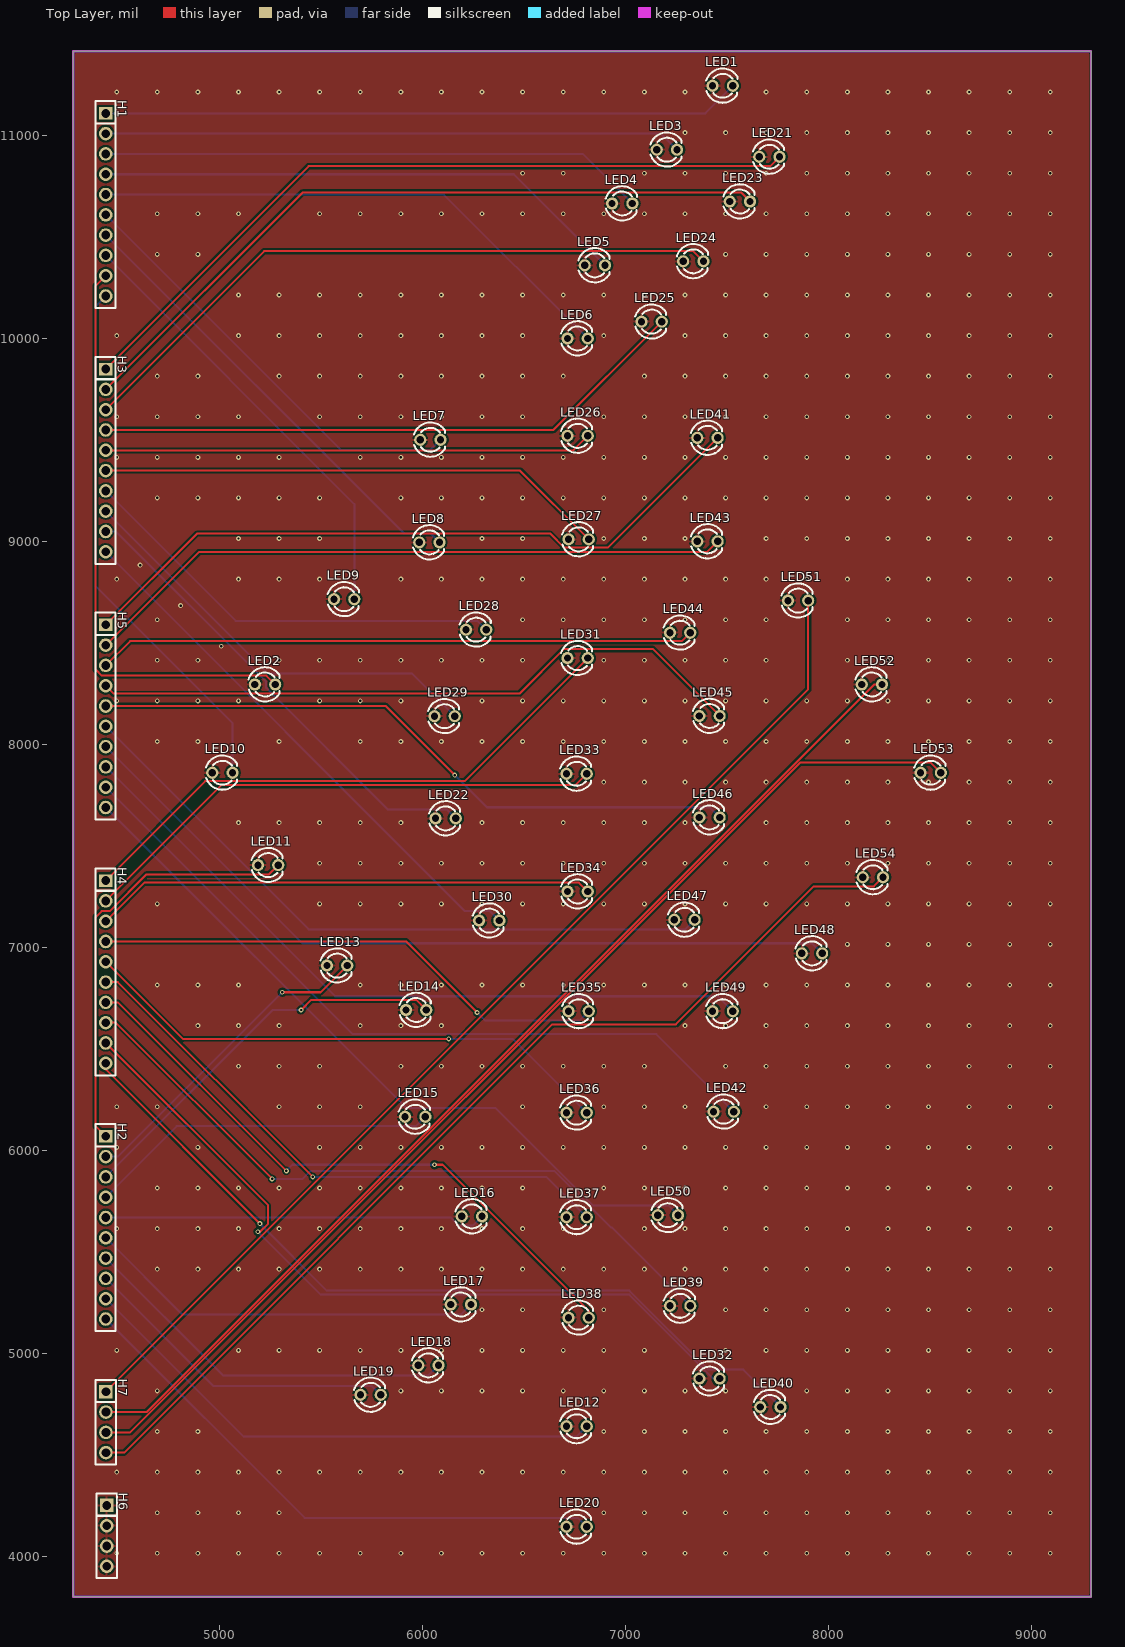
[diagram p0: Top Layer view]
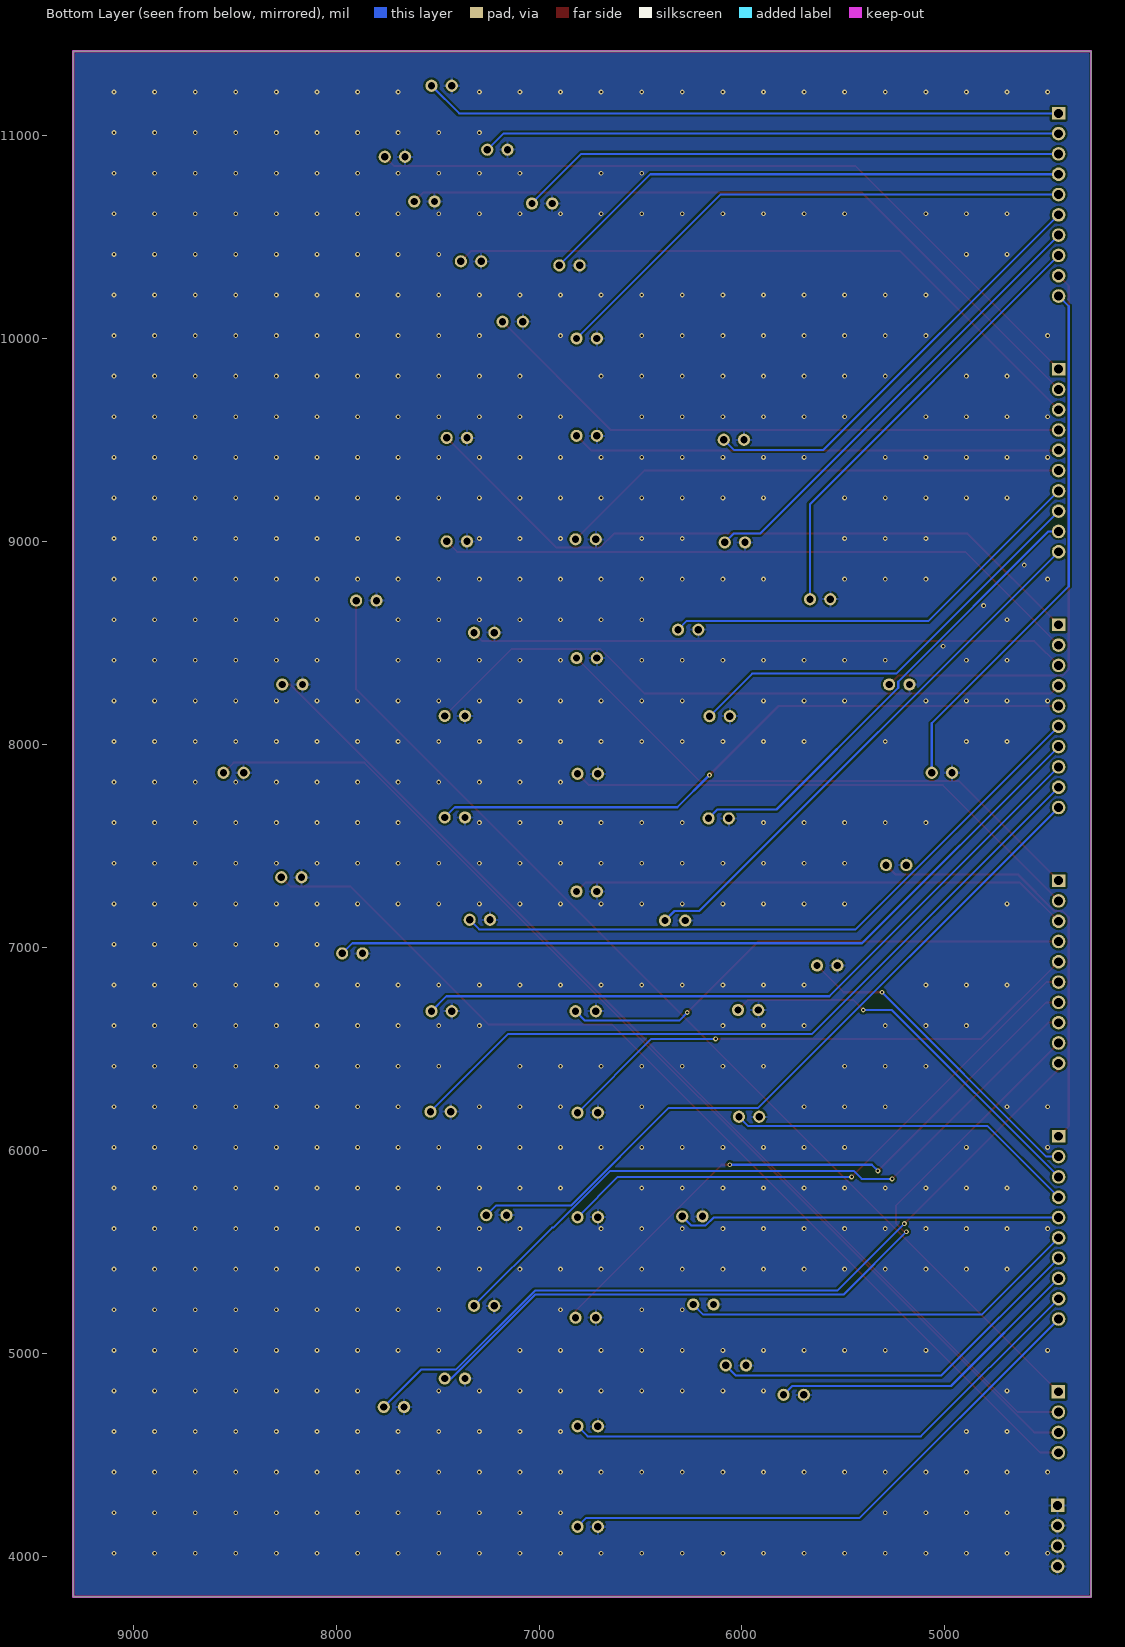
[diagram p1: Bottom Layer view, seen from below]
# Altium PCB MISC89091.pcbdoc
Units mil, origin at the board's own origin, x right, y up, seen from the top; angles counter-clockwise.
Board outline 5015 x 7615 mil, 2 copper layers (Top Layer, Bottom Layer), stack 62.206 mil thick; 61 components, 55 nets, 166 pads, 702 vias.

## Layer stack, top to bottom
Top Solder Mask Layer: solder mask 0.394, Dk 3.3
Top Layer: signal copper 1.379
Dielectric1: surface 59.449, FR4, Dk 4.5
Bottom Layer: signal copper 1.378
Bottom Solder Mask Layer: solder mask 0.394, Dk 3.3

## Board outline
4280,11415 4280,3800 9295,3800 9295,11415

## Design rules (kind name [scope] priority, off if disabled: settings)
BoardOutlineClearance copperThickness2oz_1 [All] p2 off: genericclearance=7.99 ignorepadtopadclearanceinfootprint=FALSE except(0: Arc-SplitContinuation Track-SplitContinuation SMDPad-SplitContinuation THPad-SplitContinuation Via-SplitContinuation Fill-SplitContinuation Region-SplitContinuation Poly-SplitContinuation Text-SplitContinuation Hole-SplitContinuation; 5.98: Arc-CutoutEdge SMDPad-CutoutEdge THPad-CutoutEdge Via-CutoutEdge Fill-CutoutEdge Region-CutoutEdge Text-CutoutEdge; 6.93: Hole-OutlineEdge Hole-CutoutEdge; 10: Poly-OutlineEdge Poly-CutoutEdge; 11.81: Arc-OutlineEdge Track-OutlineEdge SMDPad-OutlineEdge THPad-OutlineEdge Via-OutlineEdge Fill-OutlineEdge Region-OutlineEdge Text-OutlineEdge Track-CutoutEdge)
BoardOutlineClearance copperThickness1oz_1 [All] p4: genericclearance=4.02 ignorepadtopadclearanceinfootprint=FALSE except(0: Arc-SplitContinuation Track-SplitContinuation SMDPad-SplitContinuation THPad-SplitContinuation Via-SplitContinuation Fill-SplitContinuation Region-SplitContinuation Poly-SplitContinuation Text-SplitContinuation Hole-SplitContinuation; 6: SMDPad-CutoutEdge THPad-CutoutEdge Via-CutoutEdge Fill-CutoutEdge Region-CutoutEdge Text-CutoutEdge; 6.93: Hole-OutlineEdge Hole-CutoutEdge; 10: Poly-OutlineEdge Poly-CutoutEdge; 11.8: Arc-OutlineEdge Track-OutlineEdge SMDPad-OutlineEdge THPad-OutlineEdge Via-OutlineEdge Fill-OutlineEdge Region-OutlineEdge Text-OutlineEdge; 11.81: Arc-CutoutEdge Track-CutoutEdge)
Clearance copperThickness2oz [All] p1 off: gap=7.99 ignorepadtopadclearanceinfootprint=FALSE except(5.98: SMDPad-Track SMDPad-SMDPad THPad-Track SMDPad-THPad THPad-THPad Track-Via SMDPad-Via THPad-Via Via-Via Fill-Track Region-Track Fill-SMDPad Region-SMDPad Fill-THPad Region-THPad Fill-Via Region-Via Fill-Fill Fill-Region Region-Region Arc-Track Arc-SMDPad Arc-THPad Arc-Via Fill-Arc Region-Arc Arc-Arc Text-Track SMDPad-Text Text-THPad Text-Via Fill-Text Region-Text Arc-Text Text-Text; 6.93: Hole-Track Hole-SMDPad Hole-THPad Hole-Via Fill-Hole Region-Hole Hole-Arc Hole-Text; 10: Poly-Track Poly-SMDPad Poly-THPad Poly-Via Poly-Fill Poly-Region Poly-Poly Poly-Arc Poly-Text Poly-Hole)
Clearance copperThickness1oz [All] p3: gap=4.02 ignorepadtopadclearanceinfootprint=FALSE except(5.98: SMDPad-Track SMDPad-SMDPad THPad-Track SMDPad-THPad THPad-THPad Track-Via SMDPad-Via THPad-Via Via-Via Fill-Track Region-Track Fill-SMDPad Region-SMDPad Fill-THPad Region-THPad Fill-Via Region-Via Fill-Fill Fill-Region Region-Region; 6: Arc-Track Arc-SMDPad Arc-THPad Arc-Via Fill-Arc Region-Arc Arc-Arc Text-Track SMDPad-Text Text-THPad Text-Via Fill-Text Region-Text Arc-Text Text-Text; 6.93: Hole-Track Hole-SMDPad Hole-THPad Hole-Via Fill-Hole Region-Hole Hole-Arc Hole-Text; 10: Poly-Track Poly-SMDPad Poly-THPad Poly-Via Poly-Fill Poly-Region Poly-Poly Poly-Arc Poly-Text Poly-Hole)
Creepage creepage [All] p1: checkdistance=0 ignoreinternallayers=TRUE applytopolygonpour=TRUE
DiffPairsRouting differentialPair [All] p1: maxlimit=6 minlimit=6 mostfreqgap=6 toplayer_minwidth=5 toplayer_prefwidth=10 toplayer_maxwidth=100 toplayer_mingap=6 toplayer_prefgap=6 toplayer_maxgap=6 bottomlayer_minwidth=5 bottomlayer_prefwidth=10 bottomlayer_maxwidth=100 bottomlayer_mingap=6 bottomlayer_prefgap=6 bottomlayer_maxgap=6 maxuncoupledlength=10
HoleToHoleClearance otherClearance [All] p1: gap=11.81 allowstackedmicrovias=TRUE
Length netLength [All] p1: minlimit=0 maxlimit=0
MatchedLengths netLengthTolerance [All] p1: tolerance=1000
PasteMaskExpansion pasteMaskExpansion [All] p1: expansion=0
PlaneConnect innerPlane [All] p1: planeconnectstyle=Relief reliefexpansion=20 reliefentries=4 reliefconductorwidth=10 reliefairgap=10
PolygonConnect copperRegion [(InNet('P18') OR InNet('P19'))] p1: connectstyle=Relief reliefconductorwidth=10 reliefentries=4 polygonreliefangle="90 Angle" airgapwidth=10 via.connectstyle=Relief via.reliefconductorwidth=10 via.reliefentries=4 via.polygonreliefangle="90 Angle" via.airgapwidth=10
RoutingVias viaSize [All] p1: holewidth=12.01 width=24.02 viastyle="Through Hole" minholewidth=11.81 minwidth=19.68 maxholewidth=248.03 maxwidth=393.7
SolderMaskExpansion solderMaskExpansion [IsVia] p1: expansion=-1000 istentingtop=TRUE
SolderMaskExpansion solderMaskExpansion [All] p2: expansion=2 istentingtop=FALSE
Width copperThickness2oz_2 [All] p1 off: maxlimit=100 minlimit=8 preferedwidth=10
Width copperThickness1oz_2 [All] p2: maxlimit=100 minlimit=5 preferedwidth=10

## Components (designator, comment, footprint, x,y, rotation, side; value= is the part's Value field where it differs from the comment)
H1 "" HDR-TH_10P-P2.54-V-F 4440,10658.93 r270 top
H2 "" HDR-TH_10P-P2.54-V-F 4440,5618.53 r270 top
H3 "" HDR-TH_10P-P2.54-V-F 4440,9398.83 r270 top
H4 "" HDR-TH_10P-P2.54-V-F 4440,6878.63 r270 top
H5 "" HDR-TH_10P-P2.54-V-F 4440,8138.73 r270 top
H6 "" HDR-TH_4P-P2.54-V-F 4445,4100 r270 top
H7 "" HDR-TH_4P-P2.54-V-F 4440.79,4660 r270 top
LED1 "" LED_TH-3mm 7480,11245 r0 top
LED2 "" LED_TH-3mm 5225,8295 r0 top
LED3 "" LED_TH-3mm 7205,10930 r0 top
LED4 "" LED_TH-3mm 6985,10665 r0 top
LED5 "" LED_TH-3mm 6850,10360 r0 top
LED6 "" LED_TH-3mm 6765,10000 r0 top
LED7 "" LED_TH-3mm 6039.84,9500.65 r0 top
LED8 "" LED_TH-3mm 6035,8995 r0 top
LED9 "" LED_TH-3mm 5615,8715 r0 top
LED10 "" LED_TH-3mm 5015,7860 r0 top
LED11 "" LED_TH-3mm 5240,7405 r0 top
LED12 "" LED_TH-3mm 6760,4640 r0 top
LED13 "" LED_TH-3mm 5580,6910 r0 top
LED14 "" LED_TH-3mm 5969.37,6691.15 r0 top
LED15 "" LED_TH-3mm 5965,6165 r0 top
LED16 "" LED_TH-3mm 6244.37,5674.15 r0 top
LED17 "" LED_TH-3mm 6190,5240 r0 top
LED18 "" LED_TH-3mm 6030,4940 r0 top
LED19 "" LED_TH-3mm 5745,4795 r0 top
LED20 "" LED_TH-3mm 6760,4145 r0 top
LED21 "" LED_TH-3mm 7710,10895 r0 top
LED22 "" LED_TH-3mm 6114.68,7635.14 r0 top
LED23 "" LED_TH-3mm 7564.68,10674.65 r0 top
LED24 "" LED_TH-3mm 7335,10380 r0 top
LED25 "" LED_TH-3mm 7129.68,10082.65 r0 top
LED26 "" LED_TH-3mm 6765,9520 r0 top
LED27 "" LED_TH-3mm 6770,9010 r0 top
LED28 "" LED_TH-3mm 6265,8565 r0 top
LED29 "" LED_TH-3mm 6109.68,8138.65 r0 top
LED30 "" LED_TH-3mm 6329.68,7131.64 r0 top
LED31 "" LED_TH-3mm 6765,8425 r0 top
LED32 "" LED_TH-3mm 7415,4875 r0 top
LED33 "" LED_TH-3mm 6760,7855 r0 top
LED34 "" LED_TH-3mm 6765,7275 r0 top
LED35 "" LED_TH-3mm 6770,6685 r0 top
LED36 "" LED_TH-3mm 6760,6185 r0 top
LED37 "" LED_TH-3mm 6760,5670 r0 top
LED38 "" LED_TH-3mm 6770,5175 r0 top
LED39 "" LED_TH-3mm 7270.63,5233.65 r0 top
LED40 "" LED_TH-3mm 7715,4735 r0 top
LED41 "" LED_TH-3mm 7405,9510 r0 top
LED42 "" LED_TH-3mm 7485,6190 r0 top
LED43 "" LED_TH-3mm 7405,9000 r0 top
LED44 "" LED_TH-3mm 7270,8550 r0 top
LED45 "" LED_TH-3mm 7415,8140 r0 top
LED46 "" LED_TH-3mm 7415,7640 r0 top
LED47 "" LED_TH-3mm 7291.58,7135.65 r0 top
LED48 "" LED_TH-3mm 7920,6970 r0 top
LED49 "" LED_TH-3mm 7480,6685 r0 top
LED50 "" LED_TH-3mm 7210,5680 r0 top
LED51 "" LED_TH-3mm 7851.26,8708.22 r0 top
LED52 "" LED_TH-3mm 8215,8295 r0 top
LED53 "" LED_TH-3mm 8505,7860 r0 top
LED54 "" LED_TH-3mm 8220,7345 r0 top

## Footprints (in the part's own frame and the unit in brackets; to place one, negate y for a bottom-side part, rotate by r counter-clockwise, add the part's x,y. Pads: shape width x height; smd on the part's side, far side on the other; paste and mask are expansions set on the pad)
HDR-TH_4P-P2.54-V-F [mm]
  rect 1.7x1.7 hole 1.1: 1(-3.81,0)
  round 1.7 hole 1.1: 2(-1.27,0) 3(1.27,0) 4(3.81,0)
  silkscreen extent -5.29,-1.27 5.29,1.27
HDR-TH_10P-P2.54-V-F [mm]
  rect 1.575x1.7 hole 1.1: 1(-11.43,0)
  round 1.7 hole 1.1: 2(-8.89,0) 3(-6.35,0) 4(-3.81,0) 5(-1.27,0) 6(1.27,0) 7(3.81,0) 8(6.35,0) 9(8.89,0) 10(11.43,0)
  silkscreen extent -12.95,-1.25 12.95,1.25
LED_TH-3mm [mil]
  round 60 hole 36 paste+0 mask+2: 1(-50,0) 2(50,0)
  silkscreen extent -81,-84 72,85

## Via types
v1: diameter 24.02, hole 12, Top Layer to Bottom Layer, 702 vias

## Nets (pads, with @x,y where several pads share a name; then routed paths per layer and width w, separated by ;. In a path a pad name is that pad's centre, name@x,y a point inside that pad or via, vN(x,y) a via of type N, cw(c..) or ccw(c..) an arc to the next point about the centre after c; other vN are vias at no path point)
P10: H1.1 LED1.2 | length 3146.4
  Bottom Layer w10: H1.1 7393.93,11108.93 LED1.2
P11: H1.2 LED3.2 | length 2847.7
  Bottom Layer w10: H1.2 7176.07,11008.93 LED3.2
P12: H1.3 LED4.2 | length 2696
  Bottom Layer w10: H1.3 6791.07,10908.93 LED4.2
P13: H1.4 LED5.2 | length 2646
  Bottom Layer w10: H1.4 6451.07,10808.93 LED5.2
P14: H1.5 LED6.2 | length 2668.6
  Bottom Layer w10: H1.5 6106.07,10708.93 LED6.2
P15: H1.6 LED7.2 | length 2150.3
  Bottom Layer w10: H1.6 5598.28,9450.65 6039.84,9450.65 LED7.2
P16: H1.7 LED8.2 | length 2272.1
  Bottom Layer w10: H1.7 5910,9038.93 6041.07,9038.93 LED8.2
P17: H1.8 LED9.2 | length 2201.3
  Bottom Layer w10: H1.8 5665,9183.93 LED9.2
P18: H1.9 LED2.2 | length 2876.3
  Top Layer w10: H1.9 4390,10258.93 4390,8368.94 4420,8338.94 5231.06,8338.94 LED2.2
P19: H1.10 LED10.2 | length 2649.2
  Bottom Layer w10: H1.10 4390,10158.93 4390,8778.93 5065,8103.93 LED10.2
P20: H2.1 LED11.2 | length 2106.9
  Top Layer w10: H2.1 4390,6118.53 4390,7148.52 4420,7178.52 4460,7178.52 4640,7358.52 5243.53,7358.52 LED11.2
P21: H2.2 LED13.2 | length 1580
  Top Layer w10: v1(5310,6778.53) 5498.52,6778.53 LED13.2
  Bottom Layer w10: H2.2 4500,5968.53 v1(5310,6778.53)
P22: H2.3 LED14.2 | length 1961.5
  Top Layer w10: v1(5402.62,6691.15) 5452.62,6741.15 5969.37,6741.15 LED14.2
  Bottom Layer w10: H2.3 5262.62,6691.15 v1(5402.62,6691.15)
P23: H2.4 LED15.2 | length 1739.2
  Bottom Layer w10: H2.4 4790,6118.53 5968.53,6118.53 LED15.2
P24: H2.5 LED16.2 | length 1889.8
  Bottom Layer w10: H2.5 6140,5668.53 6180,5628.53 6248.75,5628.53 LED16.2
P25: H2.6 LED17.2 | length 1977.5
  Bottom Layer w10: H2.6 4818.53,5190 6190,5190 LED17.2
P26: H2.7 LED18.2 | length 1900.3
  Bottom Layer w10: H2.7 5018.53,4890 6030,4890 LED18.2
P27: H2.8 LED19.2 | length 1592.6
  Bottom Layer w10: H2.8 4970,4838.53 5751.47,4838.53 LED19.2
P28: H2.9 LED12.2 | length 2671.8
  Bottom Layer w10: H2.9 5118.53,4590 6760,4590 LED12.2
P29: H2.10 LED20.2 | length 2794
  Bottom Layer w10: H2.10 5420,4188.53 6766.47,4188.53 LED20.2
P30: H3.1 LED21.2 | length 3753.3
  Top Layer w10: H3.1 5440,10848.83 7713.83,10848.83 LED21.2
P31: H3.2 LED23.2 | length 3594.8
  Top Layer w10: H3.2 5410,10718.83 7570.5,10718.83 LED23.2
P32: H3.3 LED24.2 | length 3289.3
  Top Layer w10: H3.3 5221.17,10430 7335,10430 LED24.2
P33: H3.4 LED25.2 | length 2960.8
  Top Layer w10: H3.4 6645.86,9548.83 LED25.2
P34: H3.5 LED26.2 | length 2404.5
  Top Layer w10: H3.5 6743.83,9448.83 LED26.2
P35: H3.6 LED27.2 | length 2520.3
  Top Layer w10: H3.6 6481.17,9348.83 LED27.2
P36: H3.7 LED28.2 | length 2158.3
  Bottom Layer w10: H3.7 5080,8608.83 6271.17,8608.83 LED28.2
P37: H3.8 LED29.2 | length 2138.1
  Bottom Layer w10: H3.8 5240,8348.83 5949.5,8348.83 LED29.2
P38: H3.9 LED22.2 | length 2327.8
  Bottom Layer w10: H3.9 4490,9048.83 5230,8308.83 5230,8278.83 5830,7678.83 6121,7678.83 LED22.2
P39: H3.10 LED30.2 | length 2692.4
  Bottom Layer w10: H3.10 6210,7178.84 6332.49,7178.84 LED30.2
P40: H4.1 LED31.2 | length 2829.1
  Top Layer w10: H4.1 4930,7818.63 6208.63,7818.63 LED31.2
P41: H4.2 LED33.2 | length 2629.5
  Top Layer w10: H4.2 5010,7798.63 6753.62,7798.63 LED33.2
P42: H4.3 LED34.2 | length 2471.8
  Top Layer w10: H4.3 4630,7318.63 6771.37,7318.63 LED34.2
P43: H4.4 LED35.2 | length 2560.8
  Top Layer w10: H4.4 5920,7028.63 v1(6270,6678.63)
  Bottom Layer w10: v1(6270,6678.63) 6310,6638.63 6773.62,6638.63 LED35.2
P44: H4.5 LED36.2 | length 2678
  Top Layer w10: H4.5 4820,6548.63 v1(6130,6548.63)
  Bottom Layer w10: v1(6130,6548.63) 6446.37,6548.63 LED36.2
P45: H4.6 LED37.2 | length 2849.9
  Top Layer w10: H4.6 4500,6828.63 v1(5460,5868.63)
  Bottom Layer w10: v1(5460,5868.63) 6611.37,5868.63 LED37.2
P46: H4.7 LED38.2 | length 3068.1
  Top Layer w10: H4.7 4500,6728.63 v1(5330,5898.63) ; v1(6060,5928.63) 6100,5928.63 6819.99,5208.63 LED38.2
  Bottom Layer w10: v1(5330,5898.63) 5360,5928.63 v1(6060,5928.63)
P47: H4.8 LED39.2 | length 3491.6
  Top Layer w10: H4.8 4490,6628.63 v1(5260,5858.63)
  Bottom Layer w10: v1(5260,5858.63) 5410,5858.63 5450,5898.63 6649.99,5898.63 6929.99,5618.63 6935.65,5618.63 LED39.2
P48: H4.9 LED32.2 | length 3862.7
  Top Layer w10: H4.9 5240,5728.63 5240,5638.63 5200,5598.63 v1(5190,5598.63)
  Bottom Layer w10: v1(5190,5598.63) 5500,5288.63 7019.99,5288.63 7433.62,4875 LED32.2
P49: H4.10 LED40.2 | length 4044.1
  Top Layer w10: H4.10 4440,6398.63 v1(5200,5638.63)
  Bottom Layer w10: v1(5200,5638.63) 5530,5308.63 7019.99,5308.63 7409.99,4918.63 7581.37,4918.63 LED40.2
P50: H5.1 LED41.2 | length 3454.6
  Top Layer w10: H5.1 4890,9038.73 6629.99,9038.73 6699.99,8968.73 6913.73,8968.73 LED41.2
P51: H5.2 LED43.2 | length 3226.8
  Top Layer w10: H5.2 4900,8948.73 7403.73,8948.73 LED43.2
P52: H5.3 LED44.2 | length 2946.8
  Top Layer w10: H5.3 4560,8508.73 7278.73,8508.73 LED44.2
P53: H5.4 LED45.2 | length 3268.9
  Top Layer w10: H5.4 4478.73,8250 6478.73,8250 6698.73,8470 7135,8470 LED45.2
P54: H5.5 LED46.2 | length 3252.3
  Top Layer w10: H5.5 5820,8188.73 v1(6160,7848.73)
  Bottom Layer w10: v1(6160,7848.73) 6318.73,7690 7415,7690 LED46.2
P55: H5.6 LED47.2 | length 3335.2
  Bottom Layer w10: H5.6 5440,7088.73 7294.67,7088.73 LED47.2
P56: H5.7 LED48.2 | length 3952
  Bottom Layer w10: H5.7 5408.73,7020 7920,7020 LED48.2
P57: H5.8 LED49.2 | length 3588.6
  Bottom Layer w10: H5.8 5570,6758.73 7456.27,6758.73 LED49.2
P58: H5.9 LED42.2 | length 3757.2
  Bottom Layer w10: H5.9 5657.03,6571.7 7153.3,6571.7 LED42.2
P59: H5.10 LED50.2 | length 3652
  Bottom Layer w10: H5.10 5920,6208.73 6360,6208.73 6839.99,5728.74 7211.27,5728.74 LED50.2
P60: H7.1 LED51.2 | length 5331.6
  Top Layer w10: H7.1 7901.26,8270.48 LED51.2
P61: H7.2 LED52.2 | length 5309.2
  Top Layer w10: H7.2 4640.79,4710 8225.78,8295 LED52.2
P62: H7.3 LED53.2 | length 5501.8
  Top Layer w10: H7.3 4560.79,4610 7860.78,7910 8505,7910 LED53.2
P63: H7.4 LED54.2 | length 5003.5
  Top Layer w10: H7.4 4530.79,4510 6640.78,6620 7249.52,6620 7929.52,7300 8225,7300 LED54.2
VCC: H6.1 H6.2 H6.3 H6.4 LED1.1 LED2.1 LED3.1 LED4.1 LED5.1 LED6.1 LED7.1 LED8.1 LED9.1 LED10.1 LED11.1 LED12.1 LED13.1 LED14.1 LED15.1 LED16.1 LED17.1 LED18.1 LED19.1 LED20.1 LED21.1 LED22.1 LED23.1 LED24.1 LED25.1 LED26.1 LED27.1 LED28.1 LED29.1 LED30.1 LED31.1 LED32.1 LED33.1 LED34.1 LED35.1 LED36.1 LED37.1 LED38.1 LED39.1 LED40.1 LED41.1 LED42.1 LED43.1 LED44.1 LED45.1 LED46.1 LED47.1 LED48.1 LED49.1 LED50.1 LED51.1 LED52.1 LED53.1 LED54.1
  other v1: 4494.1,4014.1 4694.1,4014.1 4894.1,4014.1 5094.1,4014.1 5294.1,4014.1 5494.1,4014.1 5694.1,4014.1 5894.1,4014.1 6094.1,4014.1 6294.1,4014.1 6494.1,4014.1 6694.1,4014.1 6894.1,4014.1 7094.1,4014.1 7294.1,4014.1 7494.1,4014.1 7694.1,4014.1 7894.1,4014.1 8094.1,4014.1 8294.1,4014.1 8494.1,4014.1 8694.1,4014.1 8894.1,4014.1 9094.1,4014.1 4694.1,4214.1 4894.1,4214.1 5094.1,4214.1 5294.1,4214.1 6894.1,4214.1 7094.1,4214.1 7294.1,4214.1 7494.1,4214.1 7694.1,4214.1 7894.1,4214.1 8094.1,4214.1 8294.1,4214.1 8494.1,4214.1 8694.1,4214.1 8894.1,4214.1 9094.1,4214.1 4494.1,4414.1 4694.1,4414.1 4894.1,4414.1 5094.1,4414.1 5294.1,4414.1 5494.1,4414.1 5694.1,4414.1 5894.1,4414.1 6094.1,4414.1 6294.1,4414.1 6494.1,4414.1 6694.1,4414.1 6894.1,4414.1 7094.1,4414.1 7294.1,4414.1 7494.1,4414.1 7694.1,4414.1 7894.1,4414.1 8094.1,4414.1 8294.1,4414.1 8494.1,4414.1 8694.1,4414.1 8894.1,4414.1 9094.1,4414.1 4694.1,4614.1 4894.1,4614.1 6894.1,4614.1 7094.1,4614.1 7294.1,4614.1 7494.1,4614.1 7694.1,4614.1 7894.1,4614.1 8094.1,4614.1 8294.1,4614.1 8494.1,4614.1 8694.1,4614.1 8894.1,4614.1 9094.1,4614.1 4694.1,4814.1 5894.1,4814.1 6094.1,4814.1 6294.1,4814.1 6494.1,4814.1 6694.1,4814.1 6894.1,4814.1 7094.1,4814.1 7294.1,4814.1 7494.1,4814.1 7894.1,4814.1 8094.1,4814.1 8294.1,4814.1 8494.1,4814.1 8694.1,4814.1 8894.1,4814.1 9094.1,4814.1 4494.1,5014.1 5094.1,5014.1 5294.1,5014.1 5494.1,5014.1 5694.1,5014.1 5894.1,5014.1 6094.1,5014.1 6294.1,5014.1 6494.1,5014.1 6694.1,5014.1 6894.1,5014.1 7094.1,5014.1 7494.1,5014.1 7694.1,5014.1 7894.1,5014.1 8094.1,5014.1 8294.1,5014.1 8494.1,5014.1 8694.1,5014.1 8894.1,5014.1 9094.1,5014.1 6294.1,5214.1 6494.1,5214.1 6894.1,5214.1 7494.1,5214.1 7694.1,5214.1 7894.1,5214.1 8094.1,5214.1 8294.1,5214.1 8494.1,5214.1 8694.1,5214.1 8894.1,5214.1 9094.1,5214.1 4694.1,5414.1 4894.1,5414.1 5094.1,5414.1 5294.1,5414.1 5494.1,5414.1 5694.1,5414.1 5894.1,5414.1 6094.1,5414.1 6294.1,5414.1 6494.1,5414.1 6694.1,5414.1 6894.1,5414.1 7094.1,5414.1 7294.1,5414.1 7494.1,5414.1 7694.1,5414.1 7894.1,5414.1 8094.1,5414.1 8294.1,5414.1 8494.1,5414.1 8694.1,5414.1 8894.1,5414.1 9094.1,5414.1 4494.1,5614.1 4694.1,5614.1 4894.1,5614.1 5094.1,5614.1 5294.1,5614.1 5494.1,5614.1 5694.1,5614.1 5894.1,5614.1 6094.1,5614.1 6294.1,5614.1 6494.1,5614.1 6694.1,5614.1 7094.1,5614.1 7294.1,5614.1 7494.1,5614.1 7694.1,5614.1 7894.1,5614.1 8094.1,5614.1 8294.1,5614.1 8494.1,5614.1 8694.1,5614.1 8894.1,5614.1 9094.1,5614.1 4694.1,5814.1 4894.1,5814.1 5094.1,5814.1 5294.1,5814.1 5494.1,5814.1 5694.1,5814.1 5894.1,5814.1 6094.1,5814.1 6294.1,5814.1 6494.1,5814.1 6894.1,5814.1 7094.1,5814.1 7294.1,5814.1 7494.1,5814.1 7694.1,5814.1 7894.1,5814.1 8094.1,5814.1 8294.1,5814.1 8494.1,5814.1 8694.1,5814.1 8894.1,5814.1 9094.1,5814.1 4494.1,6014.1 4894.1,6014.1 5494.1,6014.1 5694.1,6014.1 5894.1,6014.1 6094.1,6014.1 6294.1,6014.1 6494.1,6014.1 6694.1,6014.1 6894.1,6014.1 7094.1,6014.1 7294.1,6014.1 7494.1,6014.1 7694.1,6014.1 7894.1,6014.1 8094.1,6014.1 8294.1,6014.1 8494.1,6014.1 8694.1,6014.1 8894.1,6014.1 9094.1,6014.1 4494.1,6214.1 4694.1,6214.1 5294.1,6214.1 5494.1,6214.1 5694.1,6214.1 6494.1,6214.1 6894.1,6214.1 7094.1,6214.1 7294.1,6214.1 7694.1,6214.1 7894.1,6214.1 8094.1,6214.1 8294.1,6214.1 8494.1,6214.1 8694.1,6214.1 8894.1,6214.1 9094.1,6214.1 5094.1,6414.1 5294.1,6414.1 5494.1,6414.1 5894.1,6414.1 6094.1,6414.1 6294.1,6414.1 6494.1,6414.1 6694.1,6414.1 6894.1,6414.1 7094.1,6414.1 7494.1,6414.1 7694.1,6414.1 7894.1,6414.1 8094.1,6414.1 8294.1,6414.1 8494.1,6414.1 8694.1,6414.1 8894.1,6414.1 9094.1,6414.1 4894.1,6614.1 5094.1,6614.1 5294.1,6614.1 5694.1,6614.1 5894.1,6614.1 6094.1,6614.1 7294.1,6614.1 7494.1,6614.1 7694.1,6614.1 7894.1,6614.1 8094.1,6614.1 8294.1,6614.1 8494.1,6614.1 8694.1,6614.1 8894.1,6614.1 9094.1,6614.1 4694.1,6814.1 4894.1,6814.1 5094.1,6814.1 5694.1,6814.1 5894.1,6814.1 6094.1,6814.1 6294.1,6814.1 6494.1,6814.1 6694.1,6814.1 6894.1,6814.1 7094.1,6814.1 7294.1,6814.1 7494.1,6814.1 7694.1,6814.1 7894.1,6814.1 8094.1,6814.1 8294.1,6814.1 8494.1,6814.1 8694.1,6814.1 8894.1,6814.1 9094.1,6814.1 8094.1,7014.1 8294.1,7014.1 8494.1,7014.1 8694.1,7014.1 8894.1,7014.1 9094.1,7014.1 4694.1,7214.1 5494.1,7214.1 5694.1,7214.1 5894.1,7214.1 6094.1,7214.1 6294.1,7214.1 6494.1,7214.1 6694.1,7214.1 6894.1,7214.1 7094.1,7214.1 7294.1,7214.1 7494.1,7214.1 7694.1,7214.1 7894.1,7214.1 8094.1,7214.1 8294.1,7214.1 8494.1,7214.1 8694.1,7214.1 8894.1,7214.1 9094.1,7214.1 5494.1,7414.1 5694.1,7414.1 5894.1,7414.1 6094.1,7414.1 6294.1,7414.1 6494.1,7414.1 6694.1,7414.1 6894.1,7414.1 7094.1,7414.1 7294.1,7414.1 7494.1,7414.1 7694.1,7414.1 7894.1,7414.1 8094.1,7414.1 8294.1,7414.1 8494.1,7414.1 8694.1,7414.1 8894.1,7414.1 9094.1,7414.1 5094.1,7614.1 5294.1,7614.1 5494.1,7614.1 5694.1,7614.1 5894.1,7614.1 6294.1,7614.1 6494.1,7614.1 6694.1,7614.1 6894.1,7614.1 7094.1,7614.1 7294.1,7614.1 7694.1,7614.1 7894.1,7614.1 8094.1,7614.1 8294.1,7614.1 8494.1,7614.1 8694.1,7614.1 8894.1,7614.1 9094.1,7614.1 6894.1,7814.1 7094.1,7814.1 7294.1,7814.1 7494.1,7814.1 7694.1,7814.1 7894.1,7814.1 8094.1,7814.1 8294.1,7814.1 8494.1,7814.1 8694.1,7814.1 8894.1,7814.1 9094.1,7814.1 4694.1,8014.1 4894.1,8014.1 5294.1,8014.1 5694.1,8014.1 5894.1,8014.1 6094.1,8014.1 6294.1,8014.1 6494.1,8014.1 6694.1,8014.1 6894.1,8014.1 7094.1,8014.1 7294.1,8014.1 7494.1,8014.1 7694.1,8014.1 7894.1,8014.1 8094.1,8014.1 8294.1,8014.1 8494.1,8014.1 8694.1,8014.1 8894.1,8014.1 9094.1,8014.1 4494.1,8214.1 4694.1,8214.1 4894.1,8214.1 5094.1,8214.1 5494.1,8214.1 5694.1,8214.1 5894.1,8214.1 6294.1,8214.1 6494.1,8214.1 6694.1,8214.1 6894.1,8214.1 7094.1,8214.1 7294.1,8214.1 7494.1,8214.1 7694.1,8214.1 7894.1,8214.1 8094.1,8214.1 8294.1,8214.1 8494.1,8214.1 8694.1,8214.1 8894.1,8214.1 9094.1,8214.1 4694.1,8414.1 4894.1,8414.1 5294.1,8414.1 5494.1,8414.1 5694.1,8414.1 5894.1,8414.1 6094.1,8414.1 6294.1,8414.1 6494.1,8414.1 6894.1,8414.1 7094.1,8414.1 7294.1,8414.1 7494.1,8414.1 7694.1,8414.1 8094.1,8414.1 8294.1,8414.1 8494.1,8414.1 8694.1,8414.1 8894.1,8414.1 9094.1,8414.1 5009.1,8483.39 4694.1,8614.1 6494.1,8614.1 6694.1,8614.1 6894.1,8614.1 7094.1,8614.1 7294.1,8614.1 7494.1,8614.1 7694.1,8614.1 8094.1,8614.1 8294.1,8614.1 8494.1,8614.1 8694.1,8614.1 8894.1,8614.1 9094.1,8614.1 4809.1,8683.39 4494.1,8814.1 5094.1,8814.1 5294.1,8814.1 5494.1,8814.1 5894.1,8814.1 6094.1,8814.1 6294.1,8814.1 6494.1,8814.1 6694.1,8814.1 6894.1,8814.1 7094.1,8814.1 7294.1,8814.1 7494.1,8814.1 7694.1,8814.1 7894.1,8814.1 8094.1,8814.1 8294.1,8814.1 8494.1,8814.1 8694.1,8814.1 8894.1,8814.1 9094.1,8814.1 4609.1,8883.39 5094.1,9014.1 5294.1,9014.1 5494.1,9014.1 6294.1,9014.1 6494.1,9014.1 6894.1,9014.1 7094.1,9014.1 7294.1,9014.1 7694.1,9014.1 7894.1,9014.1 8094.1,9014.1 8294.1,9014.1 8494.1,9014.1 8694.1,9014.1 8894.1,9014.1 9094.1,9014.1 4694.1,9214.1 4894.1,9214.1 5094.1,9214.1 5294.1,9214.1 5494.1,9214.1 5894.1,9214.1 6094.1,9214.1 6294.1,9214.1 6494.1,9214.1 6694.1,9214.1 6894.1,9214.1 7094.1,9214.1 7294.1,9214.1 7494.1,9214.1 7694.1,9214.1 7894.1,9214.1 8094.1,9214.1 8294.1,9214.1 8494.1,9214.1 8694.1,9214.1 8894.1,9214.1 9094.1,9214.1 4494.1,9414.1 4694.1,9414.1 4894.1,9414.1 5094.1,9414.1 5294.1,9414.1 5694.1,9414.1 5894.1,9414.1 6094.1,9414.1 6294.1,9414.1 6494.1,9414.1 6694.1,9414.1 6894.1,9414.1 7094.1,9414.1 7294.1,9414.1 7494.1,9414.1 7694.1,9414.1 7894.1,9414.1 8094.1,9414.1 8294.1,9414.1 8494.1,9414.1 8694.1,9414.1 8894.1,9414.1 9094.1,9414.1 4494.1,9614.1 4694.1,9614.1 4894.1,9614.1 5094.1,9614.1 5494.1,9614.1 5694.1,9614.1 5894.1,9614.1 6094.1,9614.1 6294.1,9614.1 6494.1,9614.1 6894.1,9614.1 7094.1,9614.1 7294.1,9614.1 7494.1,9614.1 7694.1,9614.1 7894.1,9614.1 8094.1,9614.1 8294.1,9614.1 8494.1,9614.1 8694.1,9614.1 8894.1,9614.1 9094.1,9614.1 4694.1,9814.1 4894.1,9814.1 5294.1,9814.1 5494.1,9814.1 5694.1,9814.1 5894.1,9814.1 6094.1,9814.1 6294.1,9814.1 6494.1,9814.1 6694.1,9814.1 7094.1,9814.1 7294.1,9814.1 7494.1,9814.1 7694.1,9814.1 7894.1,9814.1 8094.1,9814.1 8294.1,9814.1 8494.1,9814.1 8694.1,9814.1 8894.1,9814.1 9094.1,9814.1 4494.1,10014.1 5094.1,10014.1 5294.1,10014.1 5494.1,10014.1 5694.1,10014.1 5894.1,10014.1 6094.1,10014.1 6294.1,10014.1 6494.1,10014.1 6894.1,10014.1 7294.1,10014.1 7494.1,10014.1 7694.1,10014.1 7894.1,10014.1 8094.1,10014.1 8294.1,10014.1 8494.1,10014.1 8694.1,10014.1 8894.1,10014.1 9094.1,10014.1 5094.1,10214.1 5294.1,10214.1 5494.1,10214.1 5694.1,10214.1 5894.1,10214.1 6094.1,10214.1 6294.1,10214.1 6494.1,10214.1 6694.1,10214.1 6894.1,10214.1 7094.1,10214.1 7294.1,10214.1 7494.1,10214.1 7694.1,10214.1 7894.1,10214.1 8094.1,10214.1 8294.1,10214.1 8494.1,10214.1 8694.1,10214.1 8894.1,10214.1 9094.1,10214.1 4694.1,10414.1 4894.1,10414.1 7494.1,10414.1 7694.1,10414.1 7894.1,10414.1 8094.1,10414.1 8294.1,10414.1 8494.1,10414.1 8694.1,10414.1 8894.1,10414.1 9094.1,10414.1 4694.1,10614.1 4894.1,10614.1 5094.1,10614.1 5494.1,10614.1 5694.1,10614.1 5894.1,10614.1 6094.1,10614.1 6294.1,10614.1 6494.1,10614.1 6694.1,10614.1 6894.1,10614.1 7094.1,10614.1 7294.1,10614.1 7494.1,10614.1 7694.1,10614.1 7894.1,10614.1 8094.1,10614.1 8294.1,10614.1 8494.1,10614.1 8694.1,10614.1 8894.1,10614.1 9094.1,10614.1 6494.1,10814.1 6694.1,10814.1 7094.1,10814.1 7294.1,10814.1 7494.1,10814.1 7694.1,10814.1 7894.1,10814.1 8094.1,10814.1 8294.1,10814.1 8494.1,10814.1 8694.1,10814.1 8894.1,10814.1 9094.1,10814.1 7294.1,11014.1 7494.1,11014.1 7694.1,11014.1 7894.1,11014.1 8094.1,11014.1 8294.1,11014.1 8494.1,11014.1 8694.1,11014.1 8894.1,11014.1 9094.1,11014.1 4494.1,11214.1 4694.1,11214.1 4894.1,11214.1 5094.1,11214.1 5294.1,11214.1 5494.1,11214.1 5694.1,11214.1 5894.1,11214.1 6094.1,11214.1 6294.1,11214.1 6494.1,11214.1 6694.1,11214.1 6894.1,11214.1 7094.1,11214.1 7294.1,11214.1 7694.1,11214.1 7894.1,11214.1 8094.1,11214.1 8294.1,11214.1 8494.1,11214.1 8694.1,11214.1 8894.1,11214.1 9094.1,11214.1

## Polygon pours and split planes (outlines as drawn)
VCC on Top Layer (solid, remove dead copper, pour order 0): 3000,12170 3000,3000 10380,3000 10380,12170
VCC on Bottom Layer (solid, remove dead copper, pour order 2): 3560,11820 3560,3250 9820,3250 9820,11820

## Keep-outs
Board Outline Layer:
  the board outline again, w10